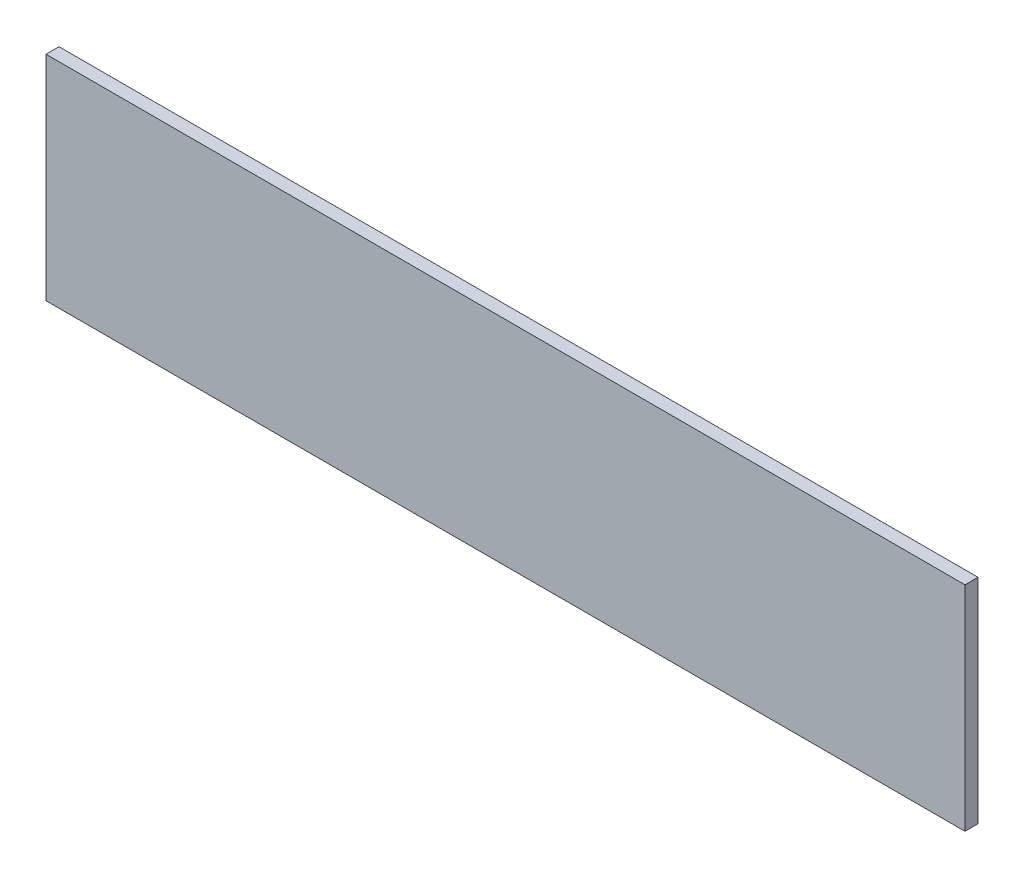
from build123d import *

# Parameters (mm, degrees)
SKETCH1_W           = 2118
SKETCH1_H           = 492
BOSS_EXTRUDE1_DEPTH = 30


with BuildPart() as part:
    # Sketch1 → Boss-Extrude1 (new body)
    with BuildSketch(Plane.XY):
        with Locations((1059, 246)):
            Rectangle(SKETCH1_W, SKETCH1_H)
    extrude(amount=BOSS_EXTRUDE1_DEPTH)


solid = part.part
